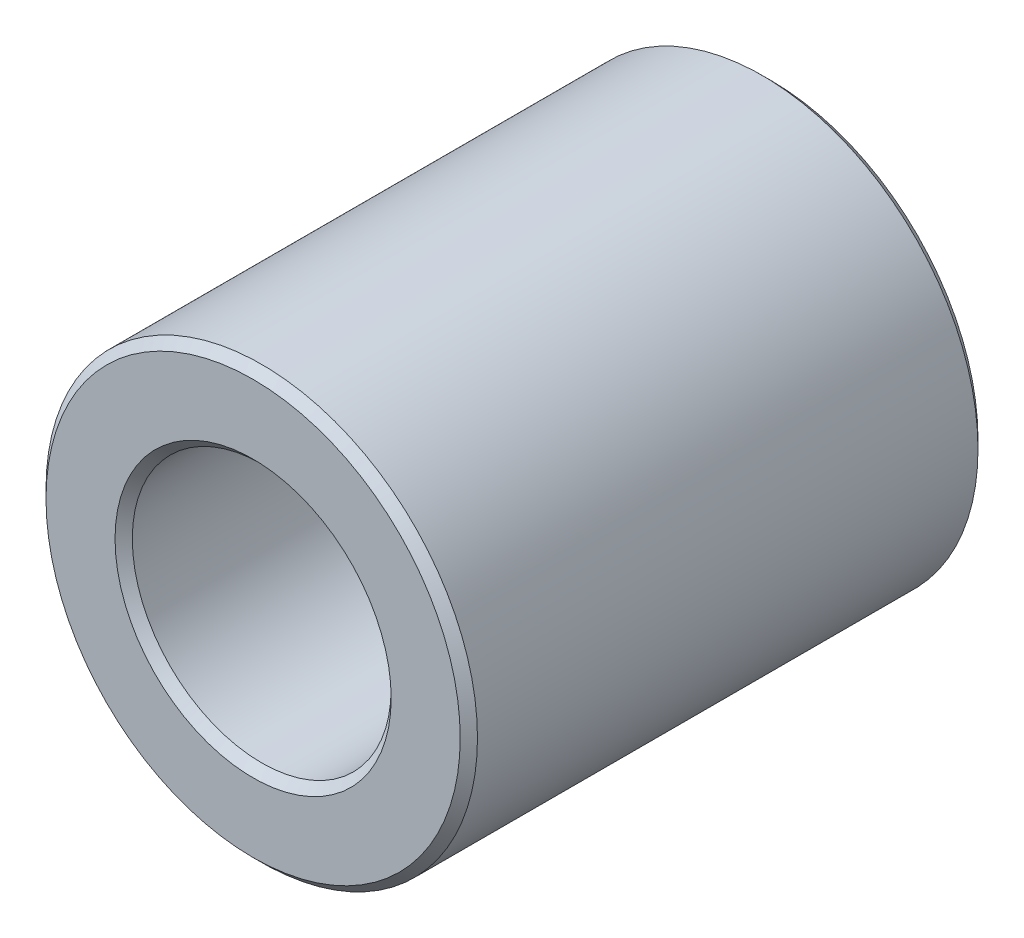
SolidWorks part; units mm, degrees
material "45#"
ref_plane "Front Plane" through (0, 0, 0) normal (0, 0, 1) x (1, 0, 0)
ref_plane "Top Plane" through (0, 0, 0) normal (0, 1, 0) x (1, 0, 0)
ref_plane "Right Plane" through (0, 0, 0) normal (1, 0, 0) x (0, 0, -1)
sketch "Sketch1" plane through (0, 0, 0) normal (0, 0, 1) x (1, 0, 0)
  circle A0 centre (0, 0) radius 25
  circle A1 centre (0, 0) radius 15
  dimension "D1" = 50
  dimension "D2" = 30
extrude "Boss-Extrude1" add sketch "Sketch1" along normal blind 60
chamfer "Chamfer1" distance 1 angle 45 4 edges at (15, 0, 0) (25, 0, 0) (15, 0, 60) (25, 0, 60)
